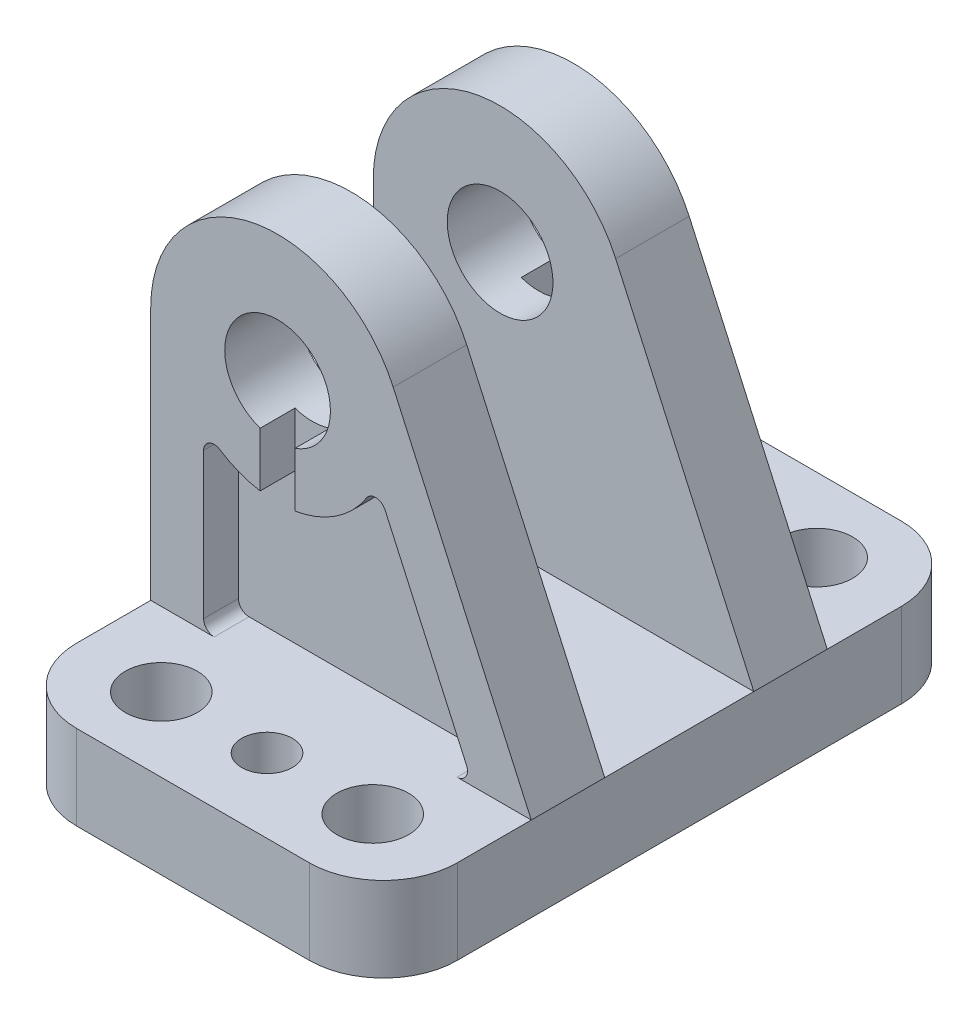
from build123d import *

# Parameters (mm, degrees)
EXTRUDE_1_DEPTH             = 6.95
SKETCH_2_W                  = 36
SKETCH_2_H                  = 6.95
EXTRUDE_2_DEPTH             = 8
SKETCH_3_W                  = 36
SKETCH_3_H                  = 8
EXTRUDE_3_DEPTH             = 14.1
EXTRUDE_4_DEPTH             = 6.95
SKETCH_5_W                  = 36
SKETCH_5_H                  = 8
EXTRUDE_5_DEPTH             = 14
CUT_EXTRUDE_1_DEPTH         = 3.3
SKETCH_7_W                  = 36
SKETCH_7_H                  = 8
EXTRUDE_6_DEPTH             = 14
CUT_EXTRUDE_START           = -3.3
CUT_EXTRUDE_2_DEPTH         = 3.3
CUT_EXTRUDE_3_DEPTH         = 3.3
CUT_EXTRUDE_4_DEPTH         = 3.3
CUT_EXTRUDE_5_DEPTH         = 4
SKETCH_12_W                 = 5
SKETCH_12_H                 = 6.95
SKETCH_13_W                 = 5
SKETCH_13_H                 = 6.95
HOLE_WIZARD_4_8_4_8_1_D     = 4.8
HOLE_WIZARD_4_8_4_8_1_DEPTH = 44
HOLE_WIZARD_6_8_6_8_1_D     = 6.8
HOLE_WIZARD_6_8_6_8_1_DEPTH = 44
FILLET_1_R                  = 1
FILLET_2_R                  = 7


with BuildPart() as part:
    # 草图1 → 凸台-拉伸1 (new body)
    with BuildSketch(Plane(origin=(0, 0, -14), x_dir=(-1, 0, 0), z_dir=(0, 0, -1))):
        with BuildLine():
            Line((-4.937253933, 36.937253933), (-18, 8))
            Line((-18, 8), (18, 8))
            Line((18, 8), (18, 32))
            ThreePointArc((18, 32), (8.525168589, 43.731305281), (-4.937253933, 36.937253933))
        make_face()
    extrude(amount=-EXTRUDE_1_DEPTH)

    # 草图2 → 凸台-拉伸2 (add)
    with BuildSketch(Plane.XZ.offset(-8)):
        with Locations((0, -10.525)):
            Rectangle(SKETCH_2_W, SKETCH_2_H)
    extrude(amount=EXTRUDE_2_DEPTH)

    # 草图3 → 凸台-拉伸3 (add)
    with BuildSketch(Plane.XY.offset(-7.05)):
        with Locations((0, 4)):
            Rectangle(SKETCH_3_W, SKETCH_3_H)
    extrude(amount=EXTRUDE_3_DEPTH)

    # 草图4 → 凸台-拉伸4 (add)
    with BuildSketch(Plane.XY.offset(7.05)):
        with BuildLine():
            Line((-18, 0), (-18, 32))
            ThreePointArc((-18, 32), (-8.525168589, 43.731305281), (4.937253933, 36.937253933))
            Line((4.937253933, 36.937253933), (18, 8))
            Line((18, 8), (18, 0))
            Line((18, 0), (-18, 0))
        make_face()
    extrude(amount=EXTRUDE_4_DEPTH)

    # 草图5 → 凸台-拉伸5 (add)
    with BuildSketch(Plane.XY.offset(14)):
        with Locations((0, 4)):
            Rectangle(SKETCH_5_W, SKETCH_5_H)
    extrude(amount=EXTRUDE_5_DEPTH)

    # 草图6 → 切除-拉伸1 (cut)
    with BuildSketch(Plane.XY.offset(14)):
        with BuildLine():
            Line((-13, 22.780455543), (-13, 8))
            Line((-13, 8), (10.965578526, 8))
            ThreePointArc((10.965578526, 8), (11.805649305, 8.457523193), (11.877016354, 9.411437828))
            Line((11.877016354, 9.411437828), (4.173334139, 26.477023221))
            ThreePointArc((4.173334139, 26.477023221), (3.334733206, 27.062929259), (2.419905737, 26.60507763))
            ThreePointArc((2.419905737, 26.60507763), (-3.895692843, 22.223912266), (-11.454545455, 23.618595948))
            ThreePointArc((-11.454545455, 23.618595948), (-12.476731295, 23.659504616), (-13, 22.780455543))
        make_face()
    extrude(amount=-CUT_EXTRUDE_1_DEPTH, mode=Mode.SUBTRACT)

    # 草图7 → 凸台-拉伸6 (add)
    with BuildSketch(Plane(origin=(0, 0, -14), x_dir=(-1, 0, 0), z_dir=(0, 0, -1))):
        with Locations((0, 4)):
            Rectangle(SKETCH_7_W, SKETCH_7_H)
    extrude(amount=EXTRUDE_6_DEPTH)

    # 草图8 → 切除-拉伸2 (cut)
    with BuildSketch(Plane(origin=(0, 0, -14), x_dir=(-1, 0, 0), z_dir=(0, 0, -1)).offset(CUT_EXTRUDE_START)):
        with BuildLine():
            Line((-4.173334139, 26.477023221), (-11.877016354, 9.411437828))
            ThreePointArc((-11.877016354, 9.411437828), (-11.805649305, 8.457523193), (-10.965578526, 8))
            Line((-10.965578526, 8), (13, 8))
            Line((13, 8), (13, 22.780455543))
            ThreePointArc((13, 22.780455543), (12.476731295, 23.659504616), (11.454545455, 23.618595948))
            ThreePointArc((11.454545455, 23.618595948), (3.895692843, 22.223912266), (-2.419905737, 26.60507763))
            ThreePointArc((-2.419905737, 26.60507763), (-3.334733206, 27.062929259), (-4.173334139, 26.477023221))
        make_face()
    extrude(amount=CUT_EXTRUDE_2_DEPTH, mode=Mode.SUBTRACT)

    # 草图9 → 切除-拉伸3 (cut)
    with BuildSketch(Plane.XY.offset(14)):
        with BuildLine():
            Line((-7.65, 27.28009534), (-7.65, 22.137064332))
            ThreePointArc((-7.65, 22.137064332), (-6, 22), (-4.35, 22.137064332))
            Line((-4.35, 22.137064332), (-4.35, 27.28009534))
            ThreePointArc((-4.35, 27.28009534), (-6, 27), (-7.65, 27.28009534))
        make_face()
    extrude(amount=-CUT_EXTRUDE_3_DEPTH, mode=Mode.SUBTRACT)

    # 草图10 → 切除-拉伸4 (cut)
    with BuildSketch(Plane(origin=(0, 0, -14), x_dir=(-1, 0, 0), z_dir=(0, 0, -1)).offset(CUT_EXTRUDE_START)):
        with BuildLine():
            Line((7.65, 22.137064332), (7.65, 27.28009534))
            ThreePointArc((7.65, 27.28009534), (6, 27), (4.35, 27.28009534))
            Line((4.35, 27.28009534), (4.35, 22.137064332))
            ThreePointArc((4.35, 22.137064332), (6, 22), (7.65, 22.137064332))
        make_face()
    extrude(amount=CUT_EXTRUDE_4_DEPTH, mode=Mode.SUBTRACT)

    # 草图11 → 切除-拉伸5 (cut)
    with BuildSketch(Plane.XZ):
        with BuildLine():
            Line((-13, 14.23538619), (-13, -14.23538619))
            ThreePointArc((-13, -14.23538619), (-8.170290449, -13.829772461), (-4.125478743, -16.5))
            Line((-4.125478743, -16.5), (4.125478743, -16.5))
            ThreePointArc((4.125478743, -16.5), (8.170290449, -13.829772461), (13, -14.23538619))
            Line((13, -14.23538619), (13, 14.23538619))
            ThreePointArc((13, 14.23538619), (8.170290449, 13.829772461), (4.125478743, 16.5))
            Line((4.125478743, 16.5), (-4.125478743, 16.5))
            ThreePointArc((-4.125478743, 16.5), (-8.170290449, 13.829772461), (-13, 14.23538619))
        make_face()
    extrude(amount=-CUT_EXTRUDE_5_DEPTH, mode=Mode.SUBTRACT)

    # 草图12 → 切除-旋转1 (revolve, cut)
    with BuildSketch(Plane(origin=(0, 32, 0), x_dir=(1, 0, 0), z_dir=(0, 1, 0))):
        with Locations((-3.5, -10.525)):
            Rectangle(SKETCH_12_W, SKETCH_12_H)
    revolve(axis=Axis((-6, 32, 7.05), (0, 0, 1)), mode=Mode.SUBTRACT)

    # 草图13 → 切除-旋转2 (revolve, cut)
    with BuildSketch(Plane.XZ.offset(-32), mode=Mode.PRIVATE) as cut_revolve_2_sk:
        with Locations((-3.5, -10.525)):
            Rectangle(SKETCH_13_W, SKETCH_13_H)
    revolve(cut_revolve_2_sk.sketch.rotate(Axis((-6, 32, -7.05), (0, 0, -1)), 180), axis=Axis((-6, 32, -7.05), (0, 0, -1)), mode=Mode.SUBTRACT)

    # Ø4.8 (4.8) 直径孔1
    with Locations(Plane(origin=(0, 0, 0), x_dir=(-1, 0, 0), z_dir=(0, -1, 0))):
        with Locations((0, 21), (0, -21)):
            Hole(HOLE_WIZARD_4_8_4_8_1_D / 2, depth=HOLE_WIZARD_4_8_4_8_1_DEPTH)

    # Ø6.8 (6.8) 直径孔1
    with Locations(Plane(origin=(0, 0, 0), x_dir=(-1, 0, 0), z_dir=(0, -1, 0))):
        with Locations((-10, 21), (-10, -21), (10, 21), (10, -21)):
            Hole(HOLE_WIZARD_6_8_6_8_1_D / 2, depth=HOLE_WIZARD_6_8_6_8_1_DEPTH)

    # 圆角1
    fillet_1_edges = [part.edges().sort_by_distance(p)[0] for p in [
        (-13, 8, -12.35),
        (-13, 2, 14.23538619),
        (-4.125478743, 2, 16.5),
        (4.125478743, 2, 16.5),
        (13, 2, 14.23538619),
        (13, 2, -14.23538619),
        (4.125478743, 2, -16.5),
        (-4.125478743, 2, -16.5),
        (-13, 2, -14.23538619),
        (-13, 8, 12.35),
    ]]
    fillet(fillet_1_edges, radius=FILLET_1_R)

    # 圆角2
    fillet_2_edges = [part.edges().sort_by_distance(p)[0] for p in [
        (-18, 4, 28),
        (18, 4, 28),
        (18, 4, -28),
        (-18, 4, -28),
    ]]
    fillet(fillet_2_edges, radius=FILLET_2_R)


solid = part.part
